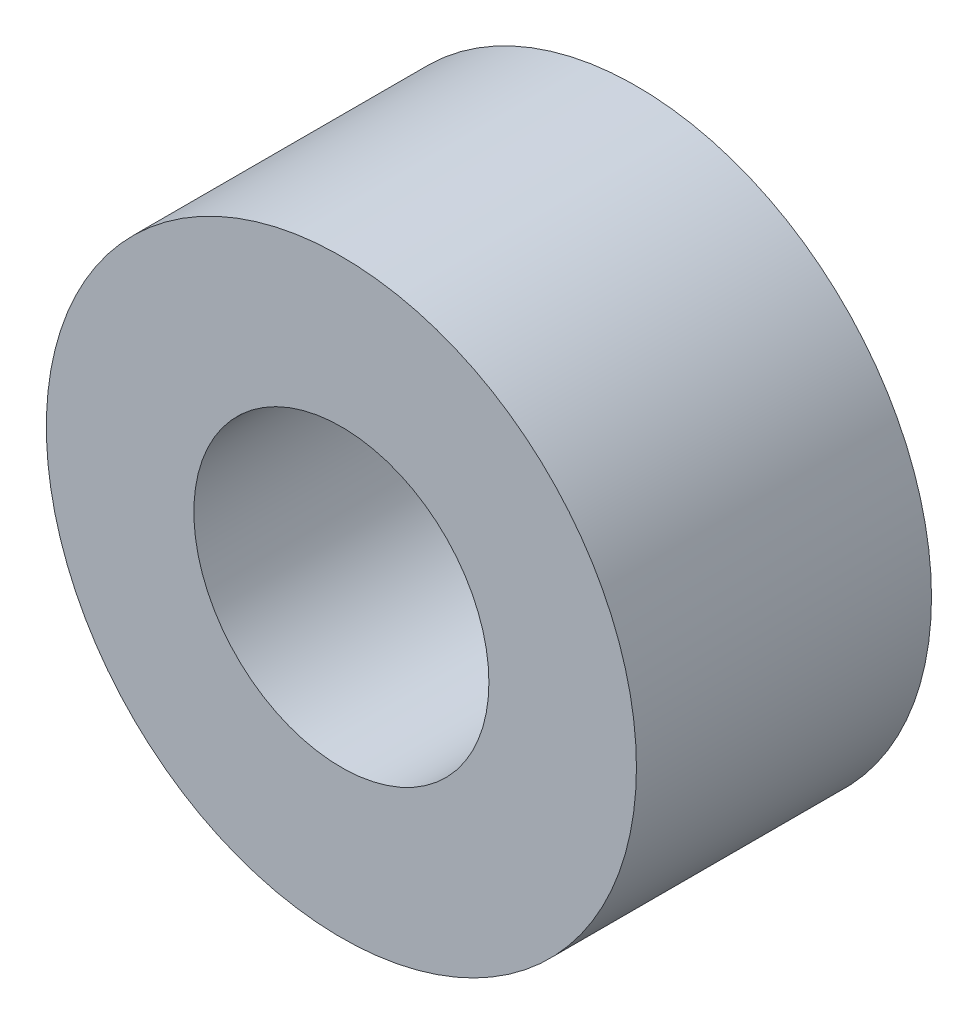
SolidWorks part; units mm, degrees
ref_plane "前视基准面" through (0, 0, 0) normal (0, 0, 1) x (1, 0, 0)
ref_plane "上视基准面" through (0, 0, 0) normal (0, 1, 0) x (1, 0, 0)
ref_plane "右视基准面" through (0, 0, 0) normal (1, 0, 0) x (0, 0, -1)
sketch "草图1" plane through (0, 0, 0) normal (0, 0, 1) x (1, 0, 0)
  circle A0 centre (0, 0) radius 20
  circle A1 centre (0, 0) radius 40
  dimension "D1" = 40
  dimension "D2" = 80
extrude "凸台-拉伸1" add sketch "草图1" along normal mid plane 40
